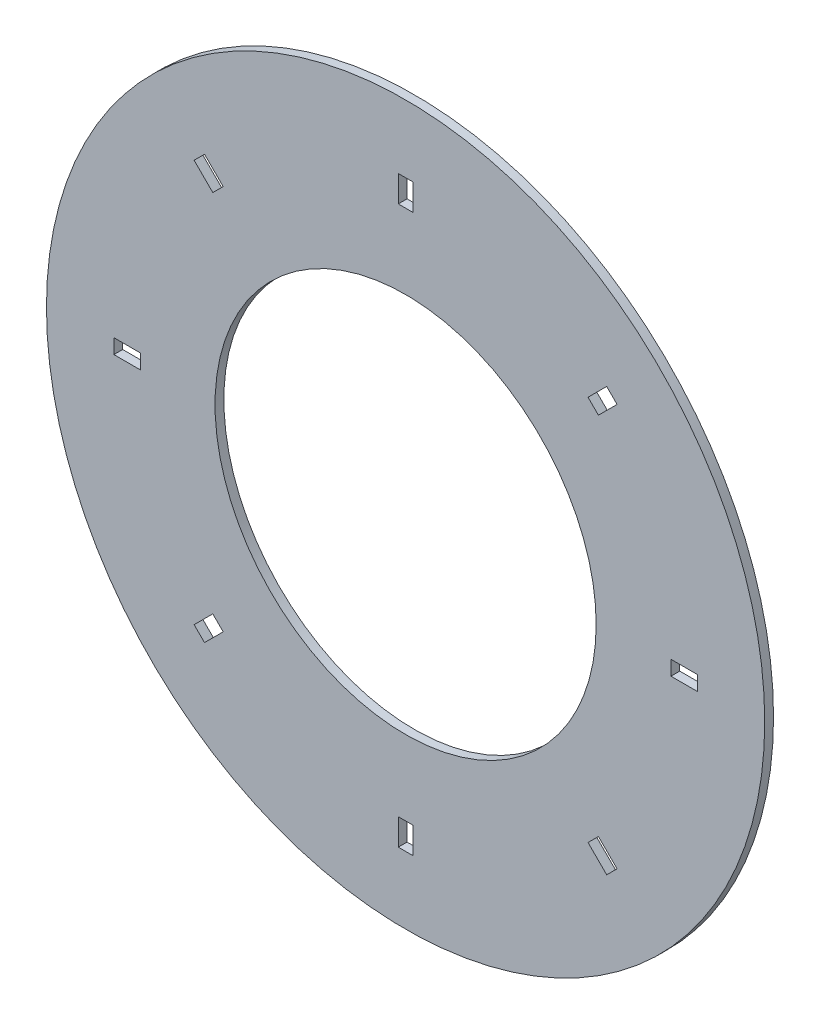
from build123d import *

# Parameters (mm, degrees)
SKETCH_1_R               = 122.5
SKETCH_1_R_2             = 65
EXTRUDE_1_DEPTH          = 3
SKETCH_2_W               = 5
SKETCH_2_H               = 9
CUT_EXTRUDE_1_DEPTH      = 5
PATTERN_CIRCULAR_1_COUNT = 8


with BuildPart() as part:
    # 草图1 → 凸台-拉伸1 (new body)
    with BuildSketch(Plane.XY):
        Circle(SKETCH_1_R)
        Circle(SKETCH_1_R_2, mode=Mode.SUBTRACT)
    extrude(amount=EXTRUDE_1_DEPTH)

    # 草图2 → 切除-拉伸1 (cut)
    with BuildSketch(Plane.XY.offset(3)):
        with Locations((0, 95)):
            Rectangle(SKETCH_2_W, SKETCH_2_H)
    cut_extrude_1 = extrude(amount=-CUT_EXTRUDE_1_DEPTH, mode=Mode.SUBTRACT)

    # 阵列(圆周)1: 切除-拉伸1 ×8 about axis
    pattern_circular_1_axis = Axis((0, 0, 0), (0, 0, 1))
    for i in range(1, PATTERN_CIRCULAR_1_COUNT):
        add(cut_extrude_1.rotate(pattern_circular_1_axis, i * 360 / PATTERN_CIRCULAR_1_COUNT), mode=Mode.SUBTRACT)


solid = part.part
